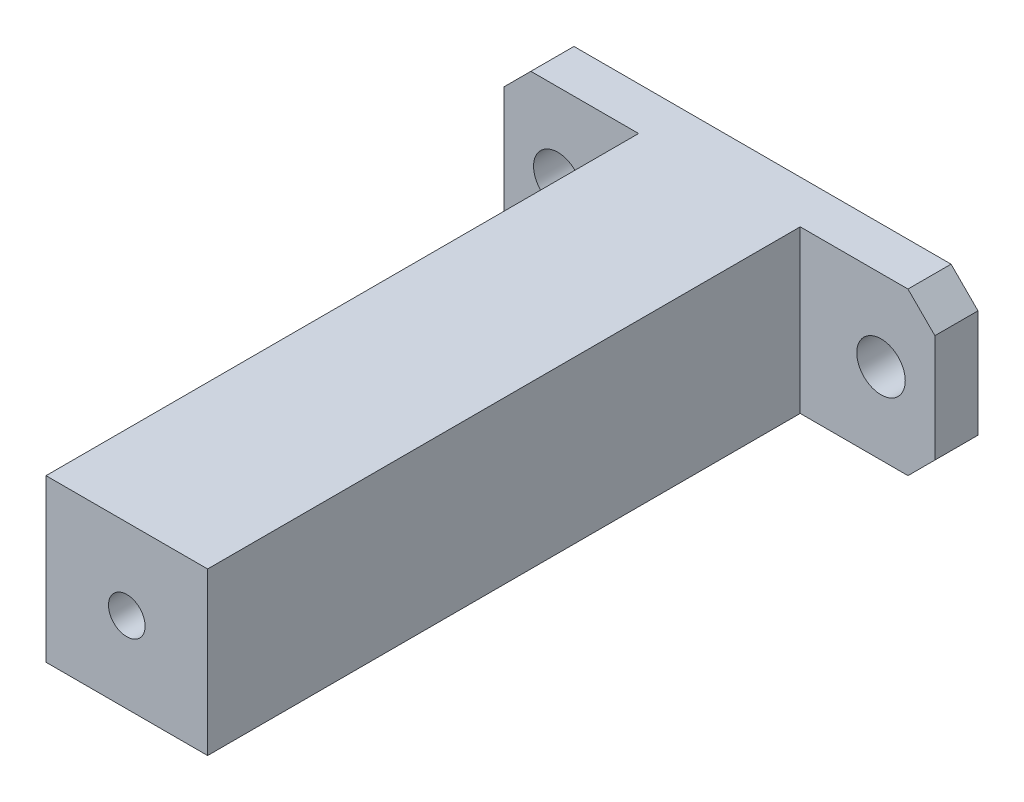
from build123d import *

# Parameters (mm, degrees)
SKETCH1_R             = 4.5
BOSS_EXTRUDE1_DEPTH   = 8
SKETCH2_W             = 30
SKETCH2_H             = 30
BOSS_EXTRUDE2_DEPTH   = 110
SKETCH3_R             = 1.5
CUT_EXTRUDE1_DEPTH    = 10
M8_TAPPED_HOLE1_D     = 6.8
M8_TAPPED_HOLE1_DEPTH = 25
M8_TAPPED_HOLE1_TIP   = 2.042926105


with BuildPart() as part:
    # Sketch1 → Boss-Extrude1 (new body)
    with BuildSketch(Plane.XY):
        Polygon((-40, 10), (-35, 15), (35, 15), (40, 10), (40, -10), (35, -15), (-35, -15), (-40, -10), align=None)
        with Locations((-30, 0)):
            Circle(SKETCH1_R, mode=Mode.SUBTRACT)
        with Locations((30, 0)):
            Circle(SKETCH1_R, mode=Mode.SUBTRACT)
    extrude(amount=BOSS_EXTRUDE1_DEPTH)

    # Sketch2 → Boss-Extrude2 (add)
    with BuildSketch(Plane.XY.offset(8)):
        Rectangle(SKETCH2_W, SKETCH2_H)
    extrude(amount=BOSS_EXTRUDE2_DEPTH)

    # Sketch3 → Cut-Extrude1 (cut)
    with BuildSketch(Plane.XY.offset(118)):
        Circle(SKETCH3_R)
    extrude(amount=-CUT_EXTRUDE1_DEPTH, mode=Mode.SUBTRACT)

    # M8 Tapped Hole1
    with Locations(Plane.XY.offset(118)):
        with Locations((0, 0)):
            Hole(M8_TAPPED_HOLE1_D / 2, depth=M8_TAPPED_HOLE1_DEPTH)
            with Locations((0, 0, -(M8_TAPPED_HOLE1_DEPTH + M8_TAPPED_HOLE1_TIP / 2))):  # 118° drill point
                Cone(0, M8_TAPPED_HOLE1_D / 2, M8_TAPPED_HOLE1_TIP, mode=Mode.SUBTRACT)


solid = part.part
